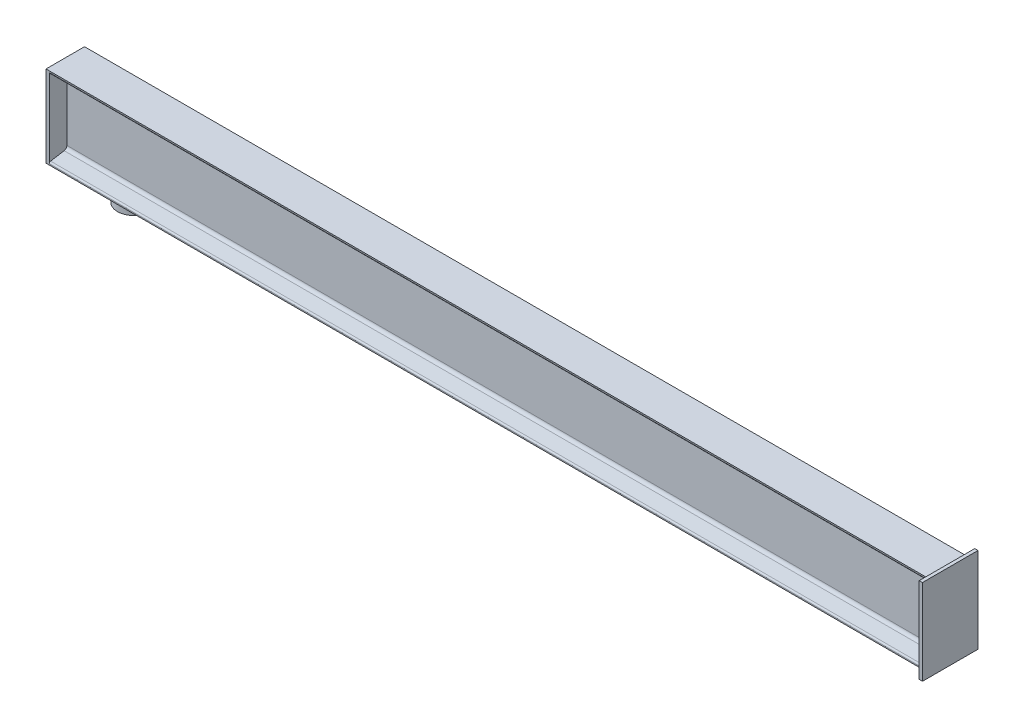
SolidWorks part; units mm, degrees
ref_plane "Front" through (0, 0, 0) normal (0, 0, 1) x (1, 0, 0)
ref_plane "Top" through (0, 0, 0) normal (0, 1, 0) x (1, 0, 0)
ref_plane "Right" through (0, 0, 0) normal (1, 0, 0) x (0, 0, -1)
other "Configuration Table"
sketch "Sketch1" plane through (0, 0, 0) normal (1, 0, 0) x (0, 0, -1)
  line L0 (-59, 0) -> (59, 0)
  line L1 (0, 106.3348) -> (0, -35.2641) construction
  line L2 (-5, 233.3333) -> (-5, 16.6667)
  line L3 (-5, 16.6667) -> (-59, 7.6667)
  line L4 (-59, 7.6667) -> (-59, 0)
  line L5 (-59, 7.6667) -> (-5, 7.6667) construction
  line L6 (-5, 7.6667) -> (-5, 16.6667) construction
  line L7 (-27, 250) -> (-27, 0) construction
  line L8 (-59, 250) -> (59, 250)
  line L9 (-59, 250) -> (-59, 242.3333)
  line L10 (-59, 242.3333) -> (-5, 233.3333)
  line L11 (-59, 242.3333) -> (-5, 242.3333) construction
  line L12 (-5, 242.3333) -> (-5, 233.3333) construction
  line L13 (-27, 13) -> (-27, 0) construction
  line L14 (-27, 250) -> (-27, 237) construction
  line L15 (59, 7.6667) -> (59, 0)
  line L16 (5, 16.6667) -> (59, 7.6667)
  line L17 (5, 233.3333) -> (5, 16.6667)
  line L18 (59, 242.3333) -> (5, 233.3333)
  line L19 (59, 250) -> (59, 242.3333)
  point P22 (0, 250)
extrude "Base" add sketch "Sketch1" along normal blind 2700
fillet "Fillet1" radius 10 4 edges at (1350, 233.3333, -5) (1350, 16.6667, -5) (1350, 16.6667, 5) (1350, 233.3333, 5)
fillet "Fillet2" radius 5 4 edges at (1350, 242.3333, 59) (1350, 7.6667, 59) (1350, 7.6667, -59) (1350, 242.3333, -59)
sketch "草图1" plane through (0, 0, 0) normal (-1, 0, 0) x (0, 0, 1)
  line L1 (-59, 250) -> (59, 250)
  line L2 (-59, 250) -> (-59, 0)
  line L3 (-59, 0) -> (59, 0)
  line L4 (59, 250) -> (59, 0)
extrude "Boss-Extrude1" add sketch "草图1" along normal mid plane 10
sketch "Sketch2" plane through (2700, 0, 0) normal (1, 0, 0) x (0, 0, -1)
  line L0 (-59, 0) -> (59, 0) construction
  line L1 (-85, 256) -> (85, 256)
  line L2 (-85, 256) -> (-85, -6)
  line L3 (-85, -6) -> (85, -6)
  line L4 (85, 256) -> (85, -6)
  line L5 (59, 250) -> (-59, 250) construction
  line L6 (59, 246.569) -> (59, 3.431) construction
  line L7 (-59, 3.431) -> (-59, 246.569) construction
  dimension "D1" = 6
  dimension "D2" = 6
  dimension "D3" = 26
  dimension "D4" = 26
extrude "Boss-Extrude2" add sketch "Sketch2" along normal mid plane 10
sketch "Sketch3" plane through (0, 0, 0) normal (0, -1, 0) x (-1, 0, 0)
  line L0 (-2705, -85) -> (-2705, 85) construction
  circle A0 centre (-205, 0) radius 50
  dimension "D1" = 2500
  dimension "D2" = 100
extrude "Boss-Extrude3" add sketch "Sketch3" along normal blind 28
equation "\"D5@Sketch1\" =  ( \"b@Sketch1\" - \"d@Sketch1\" ) /12"
equation "\"D10@Sketch1\" = \"D5@Sketch1\""
equation "\"t1@Sketch1\" = \"t@Sketch1\""
equation "\"D6@Sketch1\" =  ( \"b@Sketch1\" - \"d@Sketch1\" ) /4"
